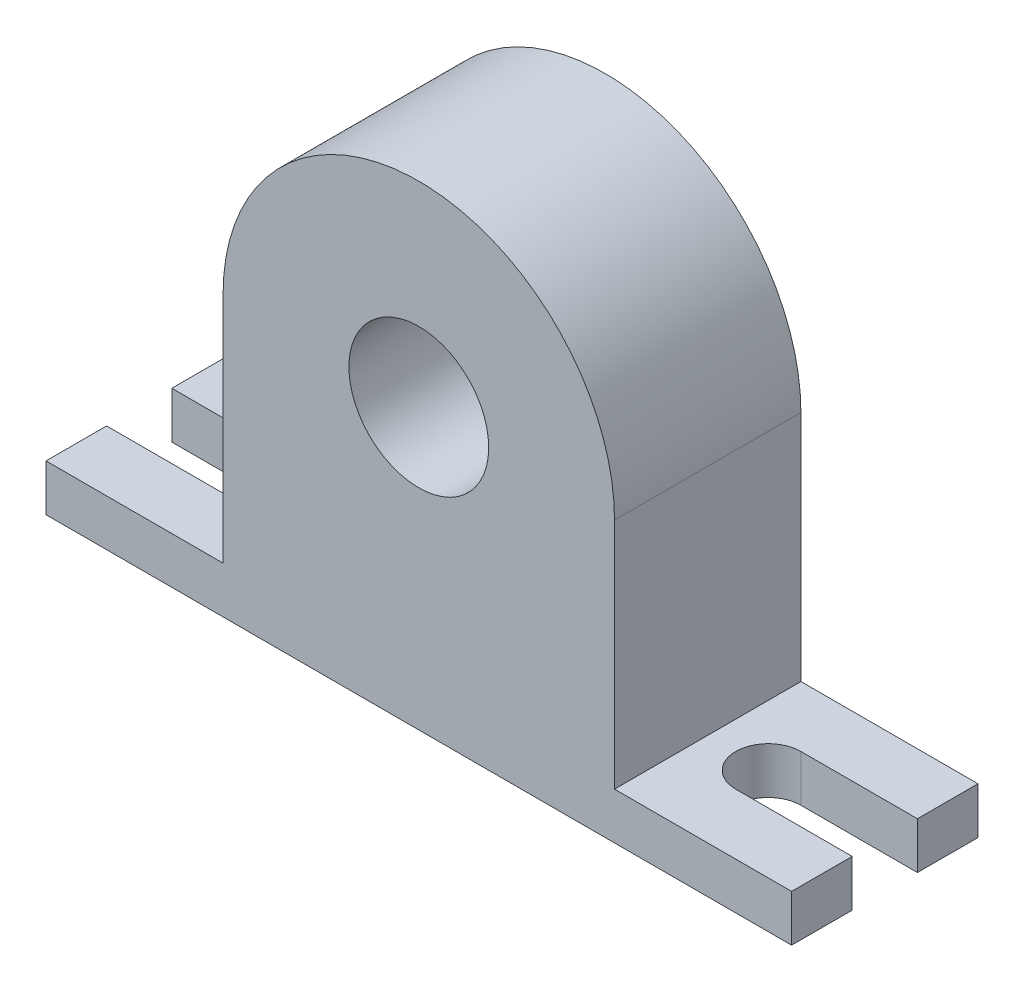
from build123d import *

# Parameters (mm, degrees)
SKETCH_1_R          = 7.5
EXTRUDE_1_DEPTH     = 20
CUT_EXTRUDE_1_DEPTH = 65.156059729


with BuildPart() as part:
    # 草图1 → 凸台-拉伸1 (new body)
    with BuildSketch(Plane.XY):
        with BuildLine():
            Line((21, 0), (21, -25))
            Line((21, -25), (40, -25))
            Line((40, -25), (40, -30))
            Line((40, -30), (21, -30))
            Line((21, -30), (-21, -30))
            Line((-21, -30), (-40, -30))
            Line((-40, -30), (-40, -25))
            Line((-40, -25), (-21, -25))
            Line((-21, -25), (-21, 0))
            ThreePointArc((-21, 0), (0, 21), (21, 0))
        make_face()
        Circle(SKETCH_1_R, mode=Mode.SUBTRACT)
    extrude(amount=EXTRUDE_1_DEPTH)

    # 草图2 → 切除-拉伸1 (cut, through all)
    with BuildSketch(Plane(origin=(0, -25, 0), x_dir=(1, 0, 0), z_dir=(0, 1, 0))):
        with BuildLine():
            Line((-27.5, -6.5), (-40, -6.5))
            Line((-40, -6.5), (-40, -13.5))
            Line((-40, -13.5), (-27.5, -13.5))
            ThreePointArc((-27.5, -13.5), (-24, -10), (-27.5, -6.5))
        make_face()
        with BuildLine():
            Line((40, -13.5), (27.5, -13.5))
            ThreePointArc((27.5, -13.5), (24, -10), (27.5, -6.5))
            Line((27.5, -6.5), (40, -6.5))
            Line((40, -6.5), (40, -13.5))
        make_face()
    extrude(amount=-CUT_EXTRUDE_1_DEPTH, mode=Mode.SUBTRACT)


solid = part.part
